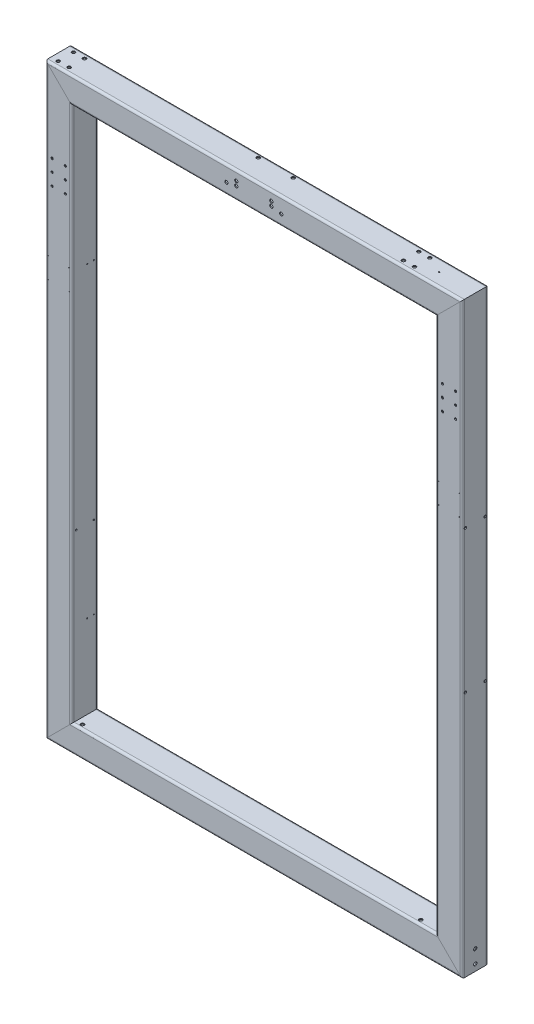
from build123d import *

# Parameters (mm, degrees)
RECTANGULAR_TUBE_120_X_80_X_8_1_DEPTH      = 1865.852813742
RECTANGULAR_TUBE_120_X_80_X_8_1_DEPTH_BACK = 85.852813742
RECTANGULAR_TUBE_120_X_80_X_8_1_2_DEPTH    = 2731.705627485
RECTANGULAR_TUBE_120_X_80_X_8_1_3_DEPTH    = 1951.705627485
RECTANGULAR_TUBE_120_X_80_X_8_1_4_DEPTH    = 2731.705627485
M12_TAPPED_HOLE1_AT_2_COUNT                = 2
M12_TAPPED_HOLE1_AT_2_PITCH                = 65
M12_TAPPED_HOLE1_AT_3_COUNT                = 2
M12_TAPPED_HOLE1_AT_3_PITCH                = 435
M12_TAPPED_HOLE1_AT_4_COUNT                = 2
M12_TAPPED_HOLE1_AT_4_PITCH                = 439.829512425
M6_TAPPED_HOLE1_AT_2_COUNT                 = 2
M6_TAPPED_HOLE1_AT_2_PITCH                 = 200.124960962
M6_TAPPED_HOLE1_AT_3_COUNT                 = 2
M6_TAPPED_HOLE1_AT_3_PITCH                 = 195.576072156
M6_TAPPED_HOLE1_AT_4_COUNT                 = 2
M6_TAPPED_HOLE1_AT_4_PITCH                 = 1215.83304775
M6_TAPPED_HOLE1_AT_5_COUNT                 = 2
M6_TAPPED_HOLE1_AT_5_PITCH                 = 1215.092589065
SKETCH9_R                                  = 5.5
SKETCH9_R_2                                = 7.5
CUT_EXTRUDE1_DEPTH                         = 10
SKETCH10_R                                 = 5
CUT_EXTRUDE2_DEPTH                         = 296
SKETCH27_R                                 = 7.5
SKETCH27_R_2                               = 1.5
CUT_EXTRUDE5_DEPTH                         = 10
SKETCH28_R                                 = 7.5
CUT_EXTRUDE6_DEPTH                         = 10
SKETCH29_R                                 = 7.5
CUT_EXTRUDE7_DEPTH                         = 10
M8_TAPPED_HOLE3_AT_2_COUNT                 = 2
M8_TAPPED_HOLE3_AT_2_PITCH                 = 80
M6_TAPPED_HOLE3_AT_2_COUNT                 = 2
M6_TAPPED_HOLE3_AT_2_PITCH                 = 30
M6_TAPPED_HOLE3_AT_3_COUNT                 = 2
M6_TAPPED_HOLE3_AT_3_PITCH                 = 1373
M6_TAPPED_HOLE3_AT_4_COUNT                 = 2
M6_TAPPED_HOLE3_AT_4_PITCH                 = 1373.327710344
SKETCH37_R                                 = 5.5
CUT_EXTRUDE8_DEPTH                         = 10
M6_TAPPED_HOLE4_AT_2_COUNT                 = 2
M6_TAPPED_HOLE4_AT_2_PITCH                 = 30
M6_TAPPED_HOLE4_AT_3_COUNT                 = 2
M6_TAPPED_HOLE4_AT_3_PITCH                 = 1400
M6_TAPPED_HOLE4_AT_4_COUNT                 = 2
M6_TAPPED_HOLE4_AT_4_PITCH                 = 1400.321391681
M8_TAPPED_HOLE4_AT_2_COUNT                 = 2
M8_TAPPED_HOLE4_AT_2_PITCH                 = 80
SKETCH43_R                                 = 7.5
CUT_EXTRUDE9_DEPTH                         = 10


with BuildPart() as part:
    # Sketch1 → Rectangular Tube 120 X 80 X 8(1) (new, two sides: drawn at the far end of the back side and taken through both)
    with BuildSketch(Plane(origin=(890, 1280, 0), x_dir=(0, -1, 0), z_dir=(-1, 0, 0)).offset(-RECTANGULAR_TUBE_120_X_80_X_8_1_DEPTH_BACK)):
        with BuildLine():
            Line((-50, -60), (50, -60))
            ThreePointArc((50, -60), (57.071067812, -57.071067812), (60, -50))
            Line((60, -50), (60, 50))
            ThreePointArc((60, 50), (57.071067812, 57.071067812), (50, 60))
            Line((50, 60), (-50, 60))
            ThreePointArc((-50, 60), (-57.071067812, 57.071067812), (-60, 50))
            Line((-60, 50), (-60, -50))
            ThreePointArc((-60, -50), (-57.071067812, -57.071067812), (-50, -60))
        make_face()
        with BuildLine():
            Line((-50, -56), (50, -56))
            ThreePointArc((50, -56), (54.242640687, -54.242640687), (56, -50))
            Line((56, -50), (56, 50))
            ThreePointArc((56, 50), (54.242640687, 54.242640687), (50, 56))
            Line((50, 56), (-50, 56))
            ThreePointArc((-50, 56), (-54.242640687, 54.242640687), (-56, 50))
            Line((-56, 50), (-56, -50))
            ThreePointArc((-56, -50), (-54.242640687, -54.242640687), (-50, -56))
        make_face(mode=Mode.SUBTRACT)
    extrude(amount=RECTANGULAR_TUBE_120_X_80_X_8_1_DEPTH + RECTANGULAR_TUBE_120_X_80_X_8_1_DEPTH_BACK)

    # Rectangular Tube 120 X 80 X 8(1) mitre 1
    split(bisect_by=Plane(origin=(890, 1280, 0), x_dir=(-0.707106781, -0.707106781, 0), z_dir=(-0.707106781, 0.707106781, 0)), keep=Keep.TOP)

    # Rectangular Tube 120 X 80 X 8(1) mitre 2
    split(bisect_by=Plane(origin=(-890, 1280, 0), x_dir=(-0.707106781, 0.707106781, 0), z_dir=(0.707106781, 0.707106781, 0)), keep=Keep.TOP)


with BuildPart() as body_2:
    # Sketch1 on segment 2 (carried to segment 2) → Rectangular Tube 120 X 80 X 8_1 2 (new body)
    with BuildSketch(Plane(origin=(-890, 1365.852813742, 0), x_dir=(1, 0, 0), z_dir=(0, -1, 0))):
        with BuildLine():
            Line((-50, -60), (50, -60))
            ThreePointArc((50, -60), (57.071067812, -57.071067812), (60, -50))
            Line((60, -50), (60, 50))
            ThreePointArc((60, 50), (57.071067812, 57.071067812), (50, 60))
            Line((50, 60), (-50, 60))
            ThreePointArc((-50, 60), (-57.071067812, 57.071067812), (-60, 50))
            Line((-60, 50), (-60, -50))
            ThreePointArc((-60, -50), (-57.071067812, -57.071067812), (-50, -60))
        make_face()
        with BuildLine():
            Line((-50, -56), (50, -56))
            ThreePointArc((50, -56), (54.242640687, -54.242640687), (56, -50))
            Line((56, -50), (56, 50))
            ThreePointArc((56, 50), (54.242640687, 54.242640687), (50, 56))
            Line((50, 56), (-50, 56))
            ThreePointArc((-50, 56), (-54.242640687, 54.242640687), (-56, 50))
            Line((-56, 50), (-56, -50))
            ThreePointArc((-56, -50), (-54.242640687, -54.242640687), (-50, -56))
        make_face(mode=Mode.SUBTRACT)
    extrude(amount=RECTANGULAR_TUBE_120_X_80_X_8_1_2_DEPTH)

    # Rectangular Tube 120 X 80 X 8_1 2 mitre
    split(bisect_by=Plane(origin=(-890, 1280, 0), x_dir=(0.707106781, -0.707106781, 0), z_dir=(-0.707106781, -0.707106781, 0)), keep=Keep.TOP)

    # Rectangular Tube 120 X 80 X 8_1 2 mi 2
    split(bisect_by=Plane(origin=(-890, -1280, 0), x_dir=(-0.707106781, -0.707106781, 0), z_dir=(-0.707106781, 0.707106781, 0)), keep=Keep.TOP)

    # Sketch6 → M12 Tapped Hole1 (revolve, cut)
    with BuildSketch(Plane(origin=(-950, 1065, -32.5), x_dir=(0, 0, 1), z_dir=(0, 1, 0))):
        Polygon((0, 0), (0, 32.314389157), (5.1, 29.25), (5.1, 0), align=None)
    m12_tapped_hole1 = revolve(axis=Axis((-956.35, 1065, -32.5), (1, 0, 0)), mode=Mode.SUBTRACT)

    # M12 Tapped Hole1 at 2: M12 Tapped Hole1 ×2
    with Locations(*[(0, 0, i * M12_TAPPED_HOLE1_AT_2_PITCH) for i in range(1, M12_TAPPED_HOLE1_AT_2_COUNT)]):
        add(m12_tapped_hole1, mode=Mode.SUBTRACT)

    # M12 Tapped Hole1 at 3: M12 Tapped Hole1 ×2
    with Locations(*[(0, -i * M12_TAPPED_HOLE1_AT_3_PITCH, 0) for i in range(1, M12_TAPPED_HOLE1_AT_3_COUNT)]):
        add(m12_tapped_hole1, mode=Mode.SUBTRACT)

    # M12 Tapped Hole1 at 4: M12 Tapped Hole1 ×2
    with Locations(*[Vector(0, -0.9890195807953914, 0.14778453506138034) * (i * M12_TAPPED_HOLE1_AT_4_PITCH) for i in range(1, M12_TAPPED_HOLE1_AT_4_COUNT)]):
        add(m12_tapped_hole1, mode=Mode.SUBTRACT)

    # Sketch8 → M6 Tapped Hole1 (revolve, cut)
    with BuildSketch(Plane(origin=(-950, 420, 0), x_dir=(0, 0, 1), z_dir=(0, 1, 0))):
        Polygon((0, 0), (0, 16.502151548), (2.5, 15), (2.5, 0), align=None)
    m6_tapped_hole1 = revolve(axis=Axis((-956.35, 420, 0), (1, 0, 0)), mode=Mode.SUBTRACT)

    # M6 Tapped Hole1 at 2: M6 Tapped Hole1 ×2
    with Locations(*[Vector(0, -0.9743911956946198, -0.2248595066987585) * (i * M6_TAPPED_HOLE1_AT_2_PITCH) for i in range(1, M6_TAPPED_HOLE1_AT_2_COUNT)]):
        add(m6_tapped_hole1, mode=Mode.SUBTRACT)

    # M6 Tapped Hole1 at 3: M6 Tapped Hole1 ×2
    with Locations(*[Vector(0, -0.9970544855015816, -0.07669649888473708) * (i * M6_TAPPED_HOLE1_AT_3_PITCH) for i in range(1, M6_TAPPED_HOLE1_AT_3_COUNT)]):
        add(m6_tapped_hole1, mode=Mode.SUBTRACT)

    # M6 Tapped Hole1 at 4: M6 Tapped Hole1 ×2
    with Locations(*[Vector(0, -0.9993148337667671, -0.037011660509880265) * (i * M6_TAPPED_HOLE1_AT_4_PITCH) for i in range(1, M6_TAPPED_HOLE1_AT_4_COUNT)]):
        add(m6_tapped_hole1, mode=Mode.SUBTRACT)

    # M6 Tapped Hole1 at 5: M6 Tapped Hole1 ×2
    with Locations(*[Vector(0, -0.9999238008152207, -0.01234473828166939) * (i * M6_TAPPED_HOLE1_AT_5_PITCH) for i in range(1, M6_TAPPED_HOLE1_AT_5_COUNT)]):
        add(m6_tapped_hole1, mode=Mode.SUBTRACT)


with BuildPart() as body_3:
    # Sketch1 on segment 3 (carried to segment 3) → Rectangular Tube 120 X 80 X 8_1 3 (new body)
    with BuildSketch(Plane(origin=(-975.852813742, -1280, 0), x_dir=(0, 1, 0), z_dir=(1, 0, 0))):
        with BuildLine():
            Line((-50, -60), (50, -60))
            ThreePointArc((50, -60), (57.071067812, -57.071067812), (60, -50))
            Line((60, -50), (60, 50))
            ThreePointArc((60, 50), (57.071067812, 57.071067812), (50, 60))
            Line((50, 60), (-50, 60))
            ThreePointArc((-50, 60), (-57.071067812, 57.071067812), (-60, 50))
            Line((-60, 50), (-60, -50))
            ThreePointArc((-60, -50), (-57.071067812, -57.071067812), (-50, -60))
        make_face()
        with BuildLine():
            Line((-50, -56), (50, -56))
            ThreePointArc((50, -56), (54.242640687, -54.242640687), (56, -50))
            Line((56, -50), (56, 50))
            ThreePointArc((56, 50), (54.242640687, 54.242640687), (50, 56))
            Line((50, 56), (-50, 56))
            ThreePointArc((-50, 56), (-54.242640687, 54.242640687), (-56, 50))
            Line((-56, 50), (-56, -50))
            ThreePointArc((-56, -50), (-54.242640687, -54.242640687), (-50, -56))
        make_face(mode=Mode.SUBTRACT)
    extrude(amount=RECTANGULAR_TUBE_120_X_80_X_8_1_3_DEPTH)

    # Rectangular Tube 120 X 80 X 8_1 3 mitre
    split(bisect_by=Plane(origin=(890, -1280, 0), x_dir=(0.707106781, -0.707106781, 0), z_dir=(-0.707106781, -0.707106781, 0)), keep=Keep.TOP)

    # Rectangular Tube 120 X 80 X 8_1 3 mi 2
    split(bisect_by=Plane(origin=(-890, -1280, 0), x_dir=(0.707106781, 0.707106781, 0), z_dir=(0.707106781, -0.707106781, 0)), keep=Keep.TOP)

    # Sketch28 → Cut-Extrude6 (cut)
    with BuildSketch(Plane(origin=(0, -1220, 0), x_dir=(1, 0, 0), z_dir=(0, 1, 0))):
        with Locations(Location((-801.5, -40, 0), (0, 0, 180))):
            Circle(SKETCH28_R)
        with Locations(Location((741.5, -40, 0), (0, 0, 180))):
            Circle(SKETCH28_R)
    extrude(amount=-CUT_EXTRUDE6_DEPTH, mode=Mode.SUBTRACT)


with BuildPart() as body_4:
    # Sketch1 on segment 4 (carried to segment 4) → Rectangular Tube 120 X 80 X 8_1 4 (new body)
    with BuildSketch(Plane(origin=(890, -1365.852813742, 0), x_dir=(-1, 0, 0), z_dir=(0, 1, 0))):
        with BuildLine():
            Line((-50, -60), (50, -60))
            ThreePointArc((50, -60), (57.071067812, -57.071067812), (60, -50))
            Line((60, -50), (60, 50))
            ThreePointArc((60, 50), (57.071067812, 57.071067812), (50, 60))
            Line((50, 60), (-50, 60))
            ThreePointArc((-50, 60), (-57.071067812, 57.071067812), (-60, 50))
            Line((-60, 50), (-60, -50))
            ThreePointArc((-60, -50), (-57.071067812, -57.071067812), (-50, -60))
        make_face()
        with BuildLine():
            Line((-50, -56), (50, -56))
            ThreePointArc((50, -56), (54.242640687, -54.242640687), (56, -50))
            Line((56, -50), (56, 50))
            ThreePointArc((56, 50), (54.242640687, 54.242640687), (50, 56))
            Line((50, 56), (-50, 56))
            ThreePointArc((-50, 56), (-54.242640687, 54.242640687), (-56, 50))
            Line((-56, 50), (-56, -50))
            ThreePointArc((-56, -50), (-54.242640687, -54.242640687), (-50, -56))
        make_face(mode=Mode.SUBTRACT)
    extrude(amount=RECTANGULAR_TUBE_120_X_80_X_8_1_4_DEPTH)

    # Rectangular Tube 120 X 80 X 8_1 4 mitre
    split(bisect_by=Plane(origin=(890, 1280, 0), x_dir=(0.707106781, 0.707106781, 0), z_dir=(0.707106781, -0.707106781, 0)), keep=Keep.TOP)

    # Rectangular Tube 120 X 80 X 8_1 4 mi 2
    split(bisect_by=Plane(origin=(890, -1280, 0), x_dir=(-0.707106781, 0.707106781, 0), z_dir=(0.707106781, 0.707106781, 0)), keep=Keep.TOP)

    # Sketch9 → Cut-Extrude1 (cut)
    with BuildSketch(Plane(origin=(950, 0, 0), x_dir=(0, 0, -1), z_dir=(1, 0, 0))):
        with Locations(Location((-45, 435, 0), (0, 0, 155.380022671))):
            Circle(SKETCH9_R)
        with Locations(Location((45, 435, 0), (0, 0, 24.619977329))):
            Circle(SKETCH9_R)
        with Locations(Location((-45, -215, 0), (0, 0, 155.380022671))):
            Circle(SKETCH9_R)
        with Locations(Location((45, -215, 0), (0, 0, 24.619977329))):
            Circle(SKETCH9_R)
        with Locations(Location((0, -1250, 0), (0, 0, 90))):
            Circle(SKETCH9_R_2)
        with Locations(Location((0, -1310, 0), (0, 0, 90))):
            Circle(SKETCH9_R_2)
    extrude(amount=-CUT_EXTRUDE1_DEPTH, mode=Mode.SUBTRACT)


with BuildPart() as cut_extrude2_tool:
    # Sketch10 → Cut-Extrude2 (new body)
    with BuildSketch(Plane.XY.offset(60)):
        with Locations((-920, 967)):
            Circle(SKETCH10_R)
        with Locations((-860, 967)):
            Circle(SKETCH10_R)
        with Locations((-920, 912)):
            Circle(SKETCH10_R)
        with Locations((-860, 912)):
            Circle(SKETCH10_R)
        with Locations((-920, 857)):
            Circle(SKETCH10_R)
        with Locations((-860, 857)):
            Circle(SKETCH10_R)
        with Locations((920, 857)):
            Circle(SKETCH10_R)
        with Locations((860, 857)):
            Circle(SKETCH10_R)
        with Locations((860, 912)):
            Circle(SKETCH10_R)
        with Locations((920, 912)):
            Circle(SKETCH10_R)
        with Locations((860, 967)):
            Circle(SKETCH10_R)
        with Locations((920, 967)):
            Circle(SKETCH10_R)
    extrude(amount=-CUT_EXTRUDE2_DEPTH)


with BuildPart() as body_2_1:
    add(body_2.part)

    # Cut-Extrude2: cut by cut_extrude2_tool
    add(cut_extrude2_tool.part, mode=Mode.SUBTRACT)


with BuildPart() as body_4_1:
    add(body_4.part)

    # Cut-Extrude2: cut by cut_extrude2_tool
    add(cut_extrude2_tool.part, mode=Mode.SUBTRACT)


with BuildPart() as cut_extrude5_tool:
    # Sketch27 → Cut-Extrude5 (new body)
    with BuildSketch(Plane.XY.offset(60)):
        with Locations((-80, 1298)):
            Circle(SKETCH27_R)
        with Locations((-80, 1278)):
            Circle(SKETCH27_R)
        with Locations((-125, 1270)):
            Circle(SKETCH27_R)
        with Locations((-937, 573)):
            Circle(SKETCH27_R_2)
        with Locations((-843, 573)):
            Circle(SKETCH27_R_2)
        with Locations((-937, 479)):
            Circle(SKETCH27_R_2)
        with Locations((-843, 479)):
            Circle(SKETCH27_R_2)
        with Locations(Location((937, 573, 0), (0, 0, 180))):
            Circle(SKETCH27_R_2)
        with Locations(Location((843, 573, 0), (0, 0, 180))):
            Circle(SKETCH27_R_2)
        with Locations(Location((843, 479, 0), (0, 0, 180))):
            Circle(SKETCH27_R_2)
        with Locations(Location((937, 479, 0), (0, 0, 180))):
            Circle(SKETCH27_R_2)
        with Locations(Location((80, 1278, 0), (0, 0, 180))):
            Circle(SKETCH27_R)
        with Locations(Location((125, 1270, 0), (0, 0, 180))):
            Circle(SKETCH27_R)
        with Locations(Location((80, 1298, 0), (0, 0, 180))):
            Circle(SKETCH27_R)
    extrude(amount=-CUT_EXTRUDE5_DEPTH)


with BuildPart() as part_1:
    add(part.part)

    # Cut-Extrude5: cut by cut_extrude5_tool
    add(cut_extrude5_tool.part, mode=Mode.SUBTRACT)

    # Sketch29 → Cut-Extrude7 (cut)
    with BuildSketch(Plane(origin=(0, 1340, 0), x_dir=(1, 0, 0), z_dir=(0, 1, 0))):
        with Locations(Location((-80, 40, 0), (0, 0, 270))):
            Circle(SKETCH29_R)
        with Locations(Location((80, 40, 0), (0, 0, 270))):
            Circle(SKETCH29_R)
        with Locations(Location((-917.5, -35, 0), (0, 0, 270))):
            Circle(SKETCH29_R)
        with Locations(Location((-867.5, -35, 0), (0, 0, 270))):
            Circle(SKETCH29_R)
        with Locations(Location((-917.5, 35, 0), (0, 0, 270))):
            Circle(SKETCH29_R)
        with Locations(Location((-867.5, 35, 0), (0, 0, 270))):
            Circle(SKETCH29_R)
        with Locations(Location((657.5, 35, 0), (0, 0, 270))):
            Circle(SKETCH29_R)
        with Locations(Location((707.5, 35, 0), (0, 0, 270))):
            Circle(SKETCH29_R)
        with Locations(Location((707.5, -35, 0), (0, 0, 270))):
            Circle(SKETCH29_R)
        with Locations(Location((657.5, -35, 0), (0, 0, 270))):
            Circle(SKETCH29_R)
    extrude(amount=-CUT_EXTRUDE7_DEPTH, mode=Mode.SUBTRACT)

    # Sketch46 → M6 Tapped Hole5 (revolve, cut)
    with BuildSketch(Plane(origin=(785, 1340, 0), x_dir=(0, 0, 1), z_dir=(1, 0, 0))):
        Polygon((0, 0), (0, 16.502151548), (2.5, 15), (2.5, 0), align=None)
    revolve(axis=Axis((785, 1346.35, 0), (0, -1, 0)), mode=Mode.SUBTRACT)


with BuildPart() as body_2_2:
    add(body_2_1.part)

    # Cut-Extrude5: cut by cut_extrude5_tool
    add(cut_extrude5_tool.part, mode=Mode.SUBTRACT)

    # Sketch40 → M6 Tapped Hole4 (revolve, cut)
    with BuildSketch(Plane(origin=(-830, -840, -10), x_dir=(0, 0, -1), z_dir=(0, 1, 0))):
        Polygon((0, 0), (0, 16.502151548), (2.5, 15), (2.5, 0), align=None)
    m6_tapped_hole4 = revolve(axis=Axis((-823.65, -840, -10), (-1, 0, 0)), mode=Mode.SUBTRACT)

    # M6 Tapped Hole4 at 2: M6 Tapped Hole4 ×2
    with Locations(*[(0, 0, -i * M6_TAPPED_HOLE4_AT_2_PITCH) for i in range(1, M6_TAPPED_HOLE4_AT_2_COUNT)]):
        add(m6_tapped_hole4, mode=Mode.SUBTRACT)

    # M6 Tapped Hole4 at 3: M6 Tapped Hole4 ×2
    with Locations(*[(0, i * M6_TAPPED_HOLE4_AT_3_PITCH, 0) for i in range(1, M6_TAPPED_HOLE4_AT_3_COUNT)]):
        add(m6_tapped_hole4, mode=Mode.SUBTRACT)

    # M6 Tapped Hole4 at 4: M6 Tapped Hole4 ×2
    with Locations(*[Vector(0, 0.9997704872016389, -0.02142365329717798) * (i * M6_TAPPED_HOLE4_AT_4_PITCH) for i in range(1, M6_TAPPED_HOLE4_AT_4_COUNT)]):
        add(m6_tapped_hole4, mode=Mode.SUBTRACT)

    # Sketch42 → M8 Tapped Hole4 (revolve, cut)
    with BuildSketch(Plane(origin=(-830, -466, 40), x_dir=(0, 0, -1), z_dir=(0, 1, 0))):
        Polygon((0, 0), (0, 21.792926105), (3.4, 19.75), (3.4, 0), align=None)
    m8_tapped_hole4 = revolve(axis=Axis((-823.65, -466, 40), (-1, 0, 0)), mode=Mode.SUBTRACT)

    # M8 Tapped Hole4 at 2: M8 Tapped Hole4 ×2
    with Locations(*[(0, 0, -i * M8_TAPPED_HOLE4_AT_2_PITCH) for i in range(1, M8_TAPPED_HOLE4_AT_2_COUNT)]):
        add(m8_tapped_hole4, mode=Mode.SUBTRACT)


with BuildPart() as body_4_2:
    add(body_4_1.part)

    # Cut-Extrude5: cut by cut_extrude5_tool
    add(cut_extrude5_tool.part, mode=Mode.SUBTRACT)

    # Sketch34 → M8 Tapped Hole3 (revolve, cut)
    with BuildSketch(Plane(origin=(830, -493, -40), x_dir=(0, 0, 1), z_dir=(0, 1, 0))):
        Polygon((0, 0), (0, 21.792926105), (3.4, 19.75), (3.4, 0), align=None)
    m8_tapped_hole3 = revolve(axis=Axis((823.65, -493, -40), (1, 0, 0)), mode=Mode.SUBTRACT)

    # M8 Tapped Hole3 at 2: M8 Tapped Hole3 ×2
    with Locations(*[(0, 0, i * M8_TAPPED_HOLE3_AT_2_PITCH) for i in range(1, M8_TAPPED_HOLE3_AT_2_COUNT)]):
        add(m8_tapped_hole3, mode=Mode.SUBTRACT)

    # Sketch36 → M6 Tapped Hole3 (revolve, cut)
    with BuildSketch(Plane(origin=(830, -840, -40), x_dir=(0, 0, 1), z_dir=(0, 1, 0))):
        Polygon((0, 0), (0, 16.502151548), (2.5, 15), (2.5, 0), align=None)
    m6_tapped_hole3 = revolve(axis=Axis((823.65, -840, -40), (1, 0, 0)), mode=Mode.SUBTRACT)

    # M6 Tapped Hole3 at 2: M6 Tapped Hole3 ×2
    with Locations(*[(0, 0, i * M6_TAPPED_HOLE3_AT_2_PITCH) for i in range(1, M6_TAPPED_HOLE3_AT_2_COUNT)]):
        add(m6_tapped_hole3, mode=Mode.SUBTRACT)

    # M6 Tapped Hole3 at 3: M6 Tapped Hole3 ×2
    with Locations(*[(0, i * M6_TAPPED_HOLE3_AT_3_PITCH, 0) for i in range(1, M6_TAPPED_HOLE3_AT_3_COUNT)]):
        add(m6_tapped_hole3, mode=Mode.SUBTRACT)

    # M6 Tapped Hole3 at 4: M6 Tapped Hole3 ×2
    with Locations(*[Vector(0, 0.999761374985732, 0.021844749635522187) * (i * M6_TAPPED_HOLE3_AT_4_PITCH) for i in range(1, M6_TAPPED_HOLE3_AT_4_COUNT)]):
        add(m6_tapped_hole3, mode=Mode.SUBTRACT)

    # Sketch37 → Cut-Extrude8 (cut)
    with BuildSketch(Plane.ZY.offset(-830)):
        with Locations(Location((-45, 420, 0), (0, 0, 204.619977329))):
            Circle(SKETCH37_R)
        with Locations(Location((45, 420, 0), (0, 0, 335.380022671))):
            Circle(SKETCH37_R)
        with Locations(Location((-45, -230, 0), (0, 0, 204.619977329))):
            Circle(SKETCH37_R)
        with Locations(Location((45, -230, 0), (0, 0, 335.380022671))):
            Circle(SKETCH37_R)
    extrude(amount=-CUT_EXTRUDE8_DEPTH, mode=Mode.SUBTRACT)


with BuildPart() as cut_extrude9_tool:
    # Sketch43 → Cut-Extrude9 (new body)
    with BuildSketch(Plane(origin=(0, 0, -60), x_dir=(-1, 0, 0), z_dir=(0, 0, -1))):
        with Locations((-877.5, -1242.5)):
            Circle(SKETCH43_R)
        with Locations((-802.5, -1242.5)):
            Circle(SKETCH43_R)
        with Locations((-802.5, -1297.5)):
            Circle(SKETCH43_R)
        with Locations((-877.5, -1297.5)):
            Circle(SKETCH43_R)
    extrude(amount=-CUT_EXTRUDE9_DEPTH)


with BuildPart() as body_3_1:
    add(body_3.part)

    # Cut-Extrude9: cut by cut_extrude9_tool
    add(cut_extrude9_tool.part, mode=Mode.SUBTRACT)


with BuildPart() as body_4_3:
    add(body_4_2.part)

    # Cut-Extrude9: cut by cut_extrude9_tool
    add(cut_extrude9_tool.part, mode=Mode.SUBTRACT)


solid = Compound([part_1.part, body_2_2.part, body_3_1.part, body_4_3.part])
